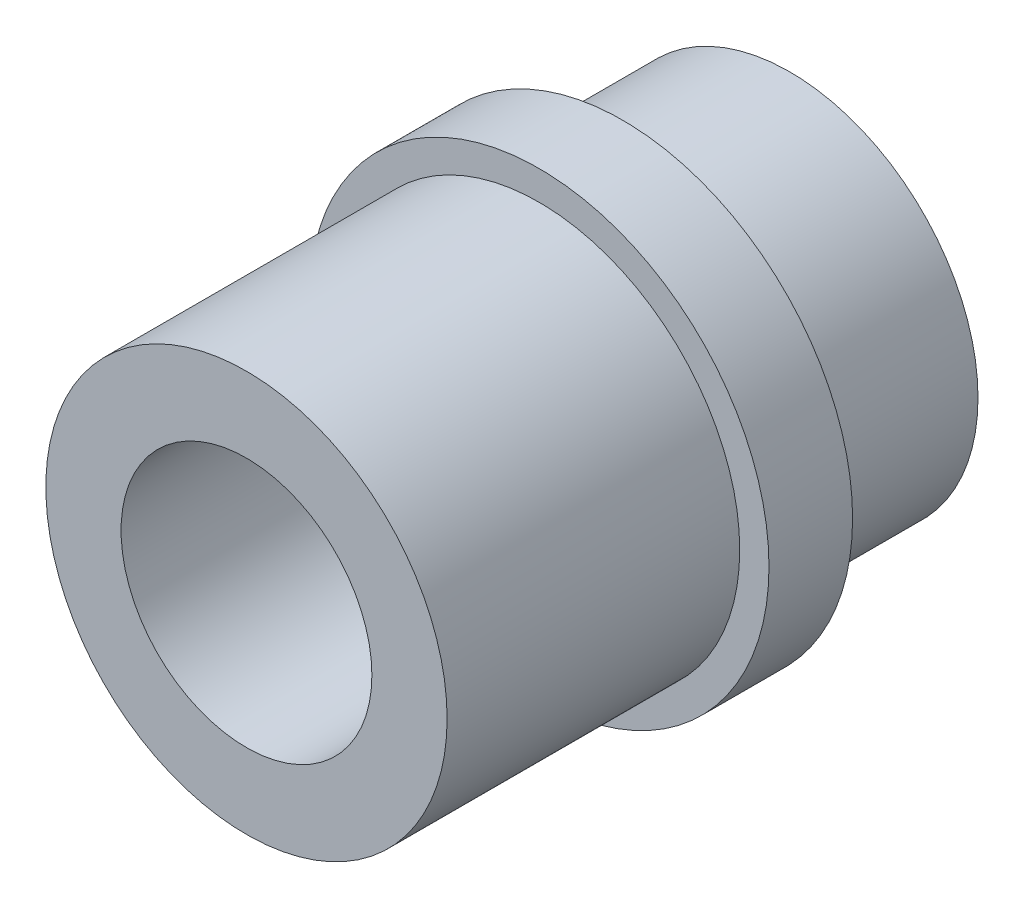
from build123d import *

# Parameters (mm, degrees)
M30X2_0_TAPPED_HOLE1_D     = 28
M30X2_0_TAPPED_HOLE1_DEPTH = 35
M30X2_0_TAPPED_HOLE1_TIP   = 8.412048666


with BuildPart() as part:
    # Sketch1 → Revolve1 (revolve)
    with BuildSketch(Plane(origin=(0, 0, 0), x_dir=(1, 0, 0), z_dir=(0, 1, 0))):
        Polygon((15, 0), (24, 0), (24, 35), (27.5, 35), (27.5, 45), (22.5, 45), (22.5, 65), (12.5, 65), (12.5, 30), (15, 30), align=None)
    revolve(axis=Axis((0, 0, 0), (0, 0, -1)))

    # M30x2.0 Tapped Hole1
    with Locations(Plane(origin=(0, 0, -65), x_dir=(-1, 0, 0), z_dir=(0, 0, -1))):
        with Locations((0, 0)):
            Hole(M30X2_0_TAPPED_HOLE1_D / 2, depth=M30X2_0_TAPPED_HOLE1_DEPTH)
            with Locations((0, 0, -(M30X2_0_TAPPED_HOLE1_DEPTH + M30X2_0_TAPPED_HOLE1_TIP / 2))):  # 118° drill point
                Cone(0, M30X2_0_TAPPED_HOLE1_D / 2, M30X2_0_TAPPED_HOLE1_TIP, mode=Mode.SUBTRACT)


solid = part.part
